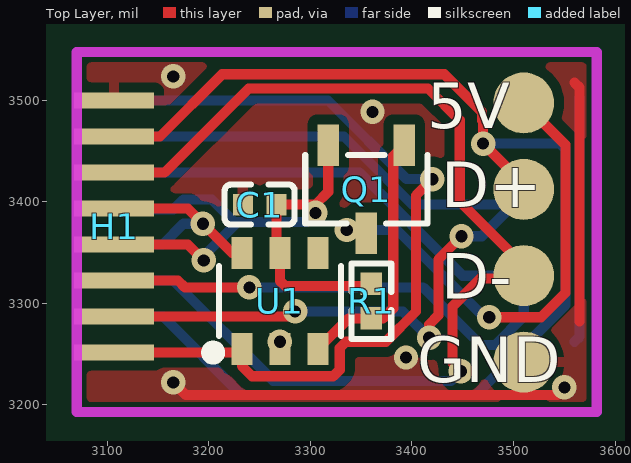
[diagram p0: Top Layer view]
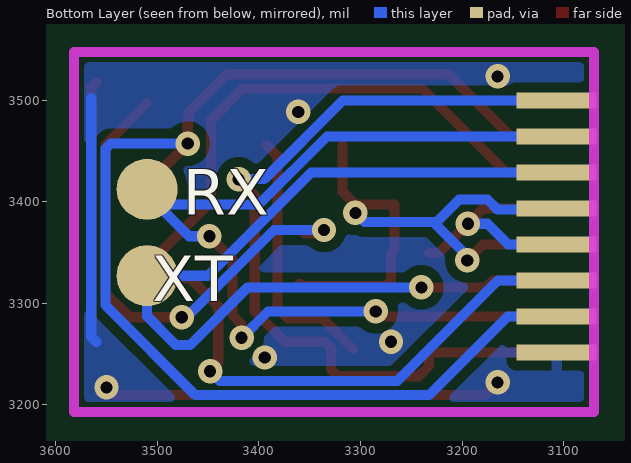
[diagram p1: Bottom Layer view, seen from below]
# Altium PCB MISC52013.pcbdoc
Units mil, origin at the board's own origin, x right, y up, seen from the top; angles counter-clockwise.
Board outline 1130 x 1092.19 mil, 2 copper layers (Top Layer, Bottom Layer), stack 62.206 mil thick; 5 components, 10 nets, 35 pads, 18 vias.

## Layer stack, top to bottom
Top Solder Mask Layer: solder mask 0.394, Dk 3.3
Top Layer: signal copper 1.379
Dielectric1: surface 59.449, FR4, Dk 4.5
Bottom Layer: signal copper 1.378
Bottom Solder Mask Layer: solder mask 0.394, Dk 3.3

## Board outline
3880,2750 2750,2750 2750,3842.19 3880,3842.19

## Design rules (kind name [scope] priority, off if disabled: settings)
BoardOutlineClearance copperThickness2oz_1 [All] p2 off: genericclearance=7.99 ignorepadtopadclearanceinfootprint=FALSE except(0: Arc-SplitContinuation Track-SplitContinuation SMDPad-SplitContinuation THPad-SplitContinuation Via-SplitContinuation Fill-SplitContinuation Region-SplitContinuation Poly-SplitContinuation Text-SplitContinuation Hole-SplitContinuation; 5.98: Arc-CutoutEdge SMDPad-CutoutEdge THPad-CutoutEdge Via-CutoutEdge Fill-CutoutEdge Region-CutoutEdge Text-CutoutEdge; 6.93: Hole-OutlineEdge Hole-CutoutEdge; 10: Poly-OutlineEdge Poly-CutoutEdge; 11.81: Arc-OutlineEdge Track-OutlineEdge SMDPad-OutlineEdge THPad-OutlineEdge Via-OutlineEdge Fill-OutlineEdge Region-OutlineEdge Text-OutlineEdge Track-CutoutEdge)
BoardOutlineClearance copperThickness1oz_1 [All] p4: genericclearance=4.02 ignorepadtopadclearanceinfootprint=FALSE except(0: SMDPad-OutlineEdge Arc-SplitContinuation Track-SplitContinuation SMDPad-SplitContinuation THPad-SplitContinuation Via-SplitContinuation Fill-SplitContinuation Region-SplitContinuation Poly-SplitContinuation Text-SplitContinuation Hole-SplitContinuation; 6: SMDPad-CutoutEdge THPad-CutoutEdge Via-CutoutEdge Fill-CutoutEdge Region-CutoutEdge Text-CutoutEdge; 6.93: Hole-OutlineEdge Hole-CutoutEdge; 10: Poly-OutlineEdge Poly-CutoutEdge; 11.8: Arc-OutlineEdge Track-OutlineEdge THPad-OutlineEdge Via-OutlineEdge Fill-OutlineEdge Region-OutlineEdge Text-OutlineEdge; 11.81: Arc-CutoutEdge Track-CutoutEdge)
Clearance copperThickness2oz [All] p1 off: gap=7.99 ignorepadtopadclearanceinfootprint=FALSE except(5.98: SMDPad-Track SMDPad-SMDPad THPad-Track SMDPad-THPad THPad-THPad Track-Via SMDPad-Via THPad-Via Via-Via Fill-Track Region-Track Fill-SMDPad Region-SMDPad Fill-THPad Region-THPad Fill-Via Region-Via Fill-Fill Fill-Region Region-Region Arc-Track Arc-SMDPad Arc-THPad Arc-Via Fill-Arc Region-Arc Arc-Arc Text-Track SMDPad-Text Text-THPad Text-Via Fill-Text Region-Text Arc-Text Text-Text; 6.93: Hole-Track Hole-SMDPad Hole-THPad Hole-Via Fill-Hole Region-Hole Hole-Arc Hole-Text; 10: Poly-Track Poly-SMDPad Poly-THPad Poly-Via Poly-Fill Poly-Region Poly-Poly Poly-Arc Poly-Text Poly-Hole)
Clearance copperThickness1oz [All] p3: gap=4.02 ignorepadtopadclearanceinfootprint=FALSE except(2: Track-Via; 5.98: SMDPad-Track SMDPad-SMDPad THPad-Track SMDPad-THPad THPad-THPad SMDPad-Via THPad-Via Via-Via Fill-Track Region-Track Fill-SMDPad Region-SMDPad Fill-THPad Region-THPad Fill-Via Region-Via Fill-Fill Fill-Region Region-Region; 6: Arc-Track Arc-SMDPad Arc-THPad Arc-Via Fill-Arc Region-Arc Arc-Arc Text-Track SMDPad-Text Text-THPad Text-Via Fill-Text Region-Text Arc-Text Text-Text; 6.93: Hole-Track Hole-SMDPad Hole-THPad Hole-Via Fill-Hole Region-Hole Hole-Arc Hole-Text; 10: Poly-Track Poly-SMDPad Poly-THPad Poly-Via Poly-Fill Poly-Region Poly-Poly Poly-Arc Poly-Text Poly-Hole)
DiffPairsRouting differentialPair [All] p1: maxlimit=6 minlimit=6 mostfreqgap=6 toplayer_minwidth=5 toplayer_prefwidth=10 toplayer_maxwidth=100 toplayer_mingap=6 toplayer_prefgap=6 toplayer_maxgap=6 bottomlayer_minwidth=5 bottomlayer_prefwidth=10 bottomlayer_maxwidth=100 bottomlayer_mingap=6 bottomlayer_prefgap=6 bottomlayer_maxgap=6 maxuncoupledlength=10
HoleToHoleClearance otherClearance [All] p1: gap=11.81 allowstackedmicrovias=TRUE
Length netLength [All] p1: minlimit=0 maxlimit=0
MatchedLengths netLengthTolerance [All] p1: tolerance=1000
PasteMaskExpansion pasteMaskExpansion [All] p1: expansion=0
PlaneConnect innerPlane [All] p1: planeconnectstyle=Relief reliefexpansion=20 reliefentries=4 reliefconductorwidth=10 reliefairgap=10
PolygonConnect copperRegion [(InNet('GND'))] p1: connectstyle=Relief reliefconductorwidth=10 reliefentries=4 polygonreliefangle="90 Angle" airgapwidth=10 via.connectstyle=Relief via.reliefconductorwidth=10 via.reliefentries=4 via.polygonreliefangle="90 Angle" via.airgapwidth=10
RoutingVias viaSize [All] p1: holewidth=12.01 width=24.02 viastyle="Through Hole" minholewidth=11.81 minwidth=19.68 maxholewidth=248.03 maxwidth=393.7
SolderMaskExpansion solderMaskExpansion [IsVia] p1: expansion=-1000 istentingtop=TRUE
SolderMaskExpansion solderMaskExpansion [All] p2: expansion=2 istentingtop=FALSE
Width copperThickness2oz_2 [All] p1 off: maxlimit=100 minlimit=8 preferedwidth=10
Width copperThickness1oz_2 [All] p2: maxlimit=100 minlimit=5 preferedwidth=10

## Components (designator, comment, footprint, x,y, rotation, side; value= is the part's Value field where it differs from the comment)
C1 "1uF" C0402 3250,3397.19 r180 top
H1 "" HDR-TH_16P-P2.54-V-F-R2-C8-S2.54-1 3106.86,3357.87 r90 top
Q1 "2301" SOT-23-3_L3.0-W1.7-P0.95-LS2.9-BR 3355,3412.19 r90 top
R1 "10K" R0402 3360,3302.19 r90 top
U1 "APS0227" TSOT-23-6_L2.9-W1.6-P0.95-LS2.8-BR 3270,3302.19 r270 top

## Footprints (in the part's own frame and the unit in brackets; to place one, negate y for a bottom-side part, rotate by r counter-clockwise, add the part's x,y. Pads: shape width x height; smd on the part's side, far side on the other; paste and mask are expansions set on the pad)
C0402 [mm]
  rect 0.5x0.54 smd: 1(-0.42,0) 2(0.42,0)
  silkscreen extent -0.87,-0.5 0.87,0.5
HDR-TH_16P-P2.54-V-F-R2-C8-S2.54-1 [mm]
  rect 0.4x2 smd: 1(-2.7,0) 3(-1.8,0) 5(-0.9,0) 7(0,0) 9(0.9,0) 11(1.8,0) 13(2.7,0) 15(3.6,0)
  rect 0.4x2 smd far side: 2(-2.7,0) 4(-1.8,0) 6(-0.9,0) 8(0,0) 10(0.9,0) 12(1.8,0) 14(2.7,0) 16(3.6,0)
R0402 [mm]
  rect 0.566x0.54 smd paste-100 mask+0.051: 1(-0.433,0) 2(0.433,0)
  silkscreen extent -0.94,-0.5 0.94,0.5
SOT-23-3_L3.0-W1.7-P0.95-LS2.9-BR [mil]
  rect 40.85x20.95 smd: 1(43.36,-37.4) 2(43.36,37.4) 3(-43.36,0)
  silkscreen extent -34,-60 34,60
TSOT-23-6_L2.9-W1.6-P0.95-LS2.8-BR [mm]
  rect 0.8x0.532 smd: 1(1.2,-0.95) 2(1.2,0) 3(1.2,0.95) 4(-1.2,0.95) 5(-1.2,0) 6(-1.2,-0.95)
  silkscreen extent -0.88,-1.82 1.44,1.53

## Free pads (board coordinates)
  round 60 smd: 1(3510,3497.19) 2(3510,3412.19) 3(3510,3327.19) 4(3510,3242.19)
  round 60 smd far side: 2(3510,3412.19) 3(3510,3327.19)

## Via types
v1: diameter 24.02, hole 12, Top Layer to Bottom Layer, 18 vias

## Nets (pads, with @x,y where several pads share a name; then routed paths per layer and width w, separated by ;. In a path a pad name is that pad's centre, name@x,y a point inside that pad or via, vN(x,y) a via of type N, cw(c..) or ccw(c..) an arc to the next point about the centre after c; other vN are vias at no path point)
$1N28: Q1.1 R1.1 U1.3 | length 255.7
  Top Layer w10: U1.3 3337.61,3285.15 R1.1 3371.61,3285.15 3381.61,3295.15 3381.61,3444.77 Q1.1
DATA1: H1.1 H1.16 U1.1 | length 840.5
  Top Layer w10: H1.1 3229.23,3251.57 U1.1 3232.6,3238.22 3242.6,3228.22 3322.42,3228.22 3328.86,3234.65 3328.86,3256.05 3335,3262.19 3374.34,3262.19 3404.02,3291.87 3404.02,3406.21 v1(3420,3422.19)
  Bottom Layer w10: H1.16 3317.41,3499.61 3394.82,3422.19 v1(3420,3422.19)
DATA2: H1.8 H1.9 U1.6 | length 239.7
  Top Layer w10: H1.9 3179.22,3393.31 v1(3194.22,3378.31) 3223.09,3349.44 U1.6
  Bottom Layer w10: H1.8 3154.57,3357.87 3175,3378.31 v1(3194.22,3378.31)
GND: C1.2 H1.2 H1.15 pad.4 U1.2 | length 872.5
  Top Layer w10: v1(3165,3222.19) 3177.53,3209.66 3542.47,3209.66 v1(3550,3217.19) ; 3560,3517.19 3565,3512.19 3565,3282.19
  Bottom Layer w10: 3560,3262.19 3565.01,3267.2 3565.01,3502.19
  other v1: 3394.13,3246.61 3270,3262.19 3361.17,3488.36 3165,3523.39
RX: H1.3 H1.14 pad.2@3510,3412.19 | length 956.5
  Top Layer w10: H1.3 3280,3287.01 v1(3285,3292.01) ; v1(3417.01,3266.02) 3417.01,3279.2 3425.98,3288.18 3425.98,3343.18 v1(3448.74,3365.94)
  Bottom Layer w10: H1.14 3333.02,3464.17 3400,3397.19 3495,3397.19 3510,3412.19 3510,3407.19 3468.74,3365.94 v1(3448.74,3365.94) ; v1(3285,3292.01) 3391.02,3292.01 v1(3417.01,3266.02)
TX: H1.5 H1.12 pad.3@3510,3327.19 | length 926.3
  Top Layer w10: H1.5 3169.75,3322.44 3176.5,3315.7 v1(3240,3315.7)
  Bottom Layer w10: H1.12 3348.45,3428.74 3450,3327.19 3510,3327.19 3510,3287.19 3481.79,3258.98 3467.64,3258.98 3410.92,3315.7 v1(3240,3315.7)
USB_D+: H1.4 H1.13 pad.2@3510,3412.19 | length 1245.8
  Top Layer w10: H1.13 3151.98,3464.17 3213.2,3525.39 3431.8,3525.39 3469.02,3488.18 3469.02,3480.22 3470,3479.23 v1(3470,3457.19) 3510,3417.19 pad.2@3510,3412.19
  Bottom Layer w10: H1.4 3155.19,3287.01 3232.53,3209.66 3462.47,3209.66 3550.98,3298.18 3550.98,3452.19 3545.98,3457.19 v1(3470,3457.19)
USB_D-: H1.6 H1.11 pad.3@3510,3327.19 | length 1102.1
  Top Layer w10: H1.11 3156.55,3428.74 3239.18,3511.38 3415.82,3511.38 3447.01,3480.19 3447.01,3400.19 3510,3337.19 3510,3327.19 3507.07,3324.26 3467.07,3324.26 3440,3297.19 3440,3241.09 v1(3447.97,3233.12)
  Bottom Layer w10: H1.6 3164.75,3322.44 3263.51,3223.68 3438.54,3223.68 v1(3447.97,3233.12)
V_5V: C1.1 H1.7 H1.10 Q1.2 R1.2 U1.5 | length 631.9
  Top Layer w10: H1.7 3179.32,3357.87 v1(3195,3342.19) ; Q1.2 3317.6,3409.79 3305,3397.19 C1.1 3266.54,3352.9 U1.5 3270,3322.19 3275,3317.19 3357.96,3317.19 R1.2
  Bottom Layer w10: H1.10 3107.98,3392.19 3165,3392.19 3175,3402.19 3202.85,3402.19 3225,3380.05 ; v1(3195,3342.19) 3195,3346.57 3225,3376.57 3225,3380.05 ; v1(3305,3389) 3296.05,3380.05 3225,3380.05
VOUT: pad.1 Q1.3 | length 485.2
  Top Layer w10: v1(3335.86,3372.19) 3339.22,3368.83 Q1.3 ; v1(3475.98,3286.21) 3526.98,3286.21 3550.98,3310.22 3550.98,3456.21 pad.1
  Bottom Layer w10: v1(3335.86,3372.19) 3385.18,3372.19 3471.16,3286.21 v1(3475.98,3286.21)
pads on no net: U1.4

## Polygon pours and split planes (outlines as drawn)
GND on Bottom Layer (solid, remove dead copper, pour order 2): 3000,3592.19 3000,3142.19 3620,3142.19 3620,3592.19
GND on Top Layer (solid, remove dead copper, pour order 0): 3041.76,3583.2 3041.76,3122.19 3630,3122.19 3630,3583.2

## Keep-outs
Board Outline Layer:
  lines w10: 3070,3192.86 3070,3547.19 3581.81,3547.19 3581.81,3192.86 3070,3192.86

## Silkscreen, mask and mechanical layers (free items; w line width, h text height)
Top Silkscreen Layer:
  text "5V" at 3415,3472.19 h45
  text "D+" at 3428.7,3394.69 h45
  text "D-" at 3428.7,3304.69 h45
  text "GND" at 3405,3222.19 h45
Bottom Silkscreen Layer:
  text "RX" at 3475,3387.19 h45
  text "TX" at 3425,3302.19 h45